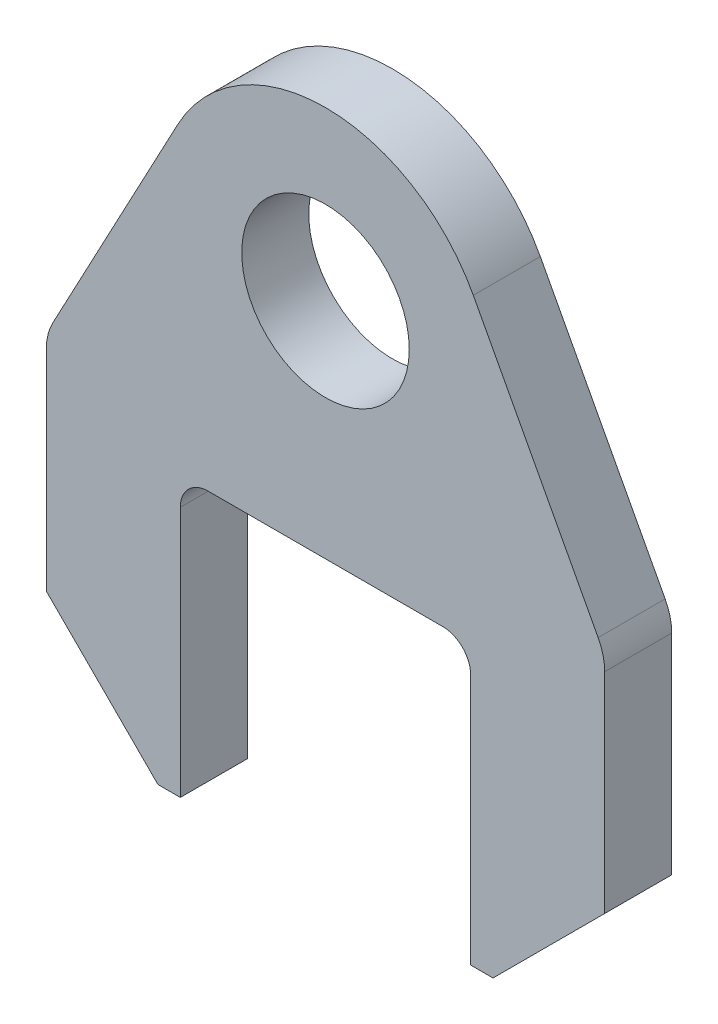
SolidWorks part; units mm, degrees
material "Q235B"
ref_plane "Front Plane" through (0, 0, 0) normal (0, 0, 1) x (1, 0, 0)
ref_plane "Top Plane" through (0, 0, 0) normal (0, 1, 0) x (1, 0, 0)
ref_plane "Right Plane" through (0, 0, 0) normal (1, 0, 0) x (0, 0, -1)
sketch "Sketch1" plane through (0, 0, 0) normal (0, 0, 1) x (1, 0, 0)
  line L0 (0, 0) -> (0, 84.1607) construction
  line L1 (-26, 0) -> (-30, 0)
  line L2 (-30, 0) -> (-50, 20)
  line L3 (-50, 20) -> (-50, 57.5)
  line L4 (-48.8235, 62.2059) -> (-26.4706, 104.1176)
  line L5 (-26, 0) -> (-26, 45)
  line L6 (-21, 50) -> (21, 50)
  line L7 (26, 0) -> (26, 45)
  line L8 (48.8235, 62.2059) -> (26.4706, 104.1176)
  line L9 (50, 20) -> (50, 57.5)
  line L10 (30, 0) -> (50, 20)
  line L11 (26, 0) -> (30, 0)
  arc A0 (-26.4706, 104.1176) -> (26.4706, 104.1176) centre (0, 90) cw
  arc A1 (48.8235, 62.2059) -> (50, 57.5) centre (40, 57.5) cw
  arc A2 (-50, 57.5) -> (-48.8235, 62.2059) centre (-40, 57.5) cw
  circle A3 centre (0, 90) radius 15
  arc A4 (26, 45) -> (21, 50) centre (21, 45) ccw
  arc A5 (-26, 45) -> (-21, 50) centre (-21, 45) cw
  point P16 (0, 50)
  point P20 (26, 50)
  point P23 (50, 60)
  point P26 (-50, 60)
  point P30 (-26, 50)
  dimension "D1" = 100
  dimension "D6" = 10
  dimension "D9" = 30
  dimension "D10" = 30
  dimension "D11" = 5
  dimension "D2" = 50
  dimension "D3" = 20
  dimension "D4" = 60
  dimension "D5" = 52
  dimension "D7" = 57.5
  dimension "D8" = 32.5
extrude "Boss-Extrude1" add sketch "Sketch1" along normal mid plane 12
